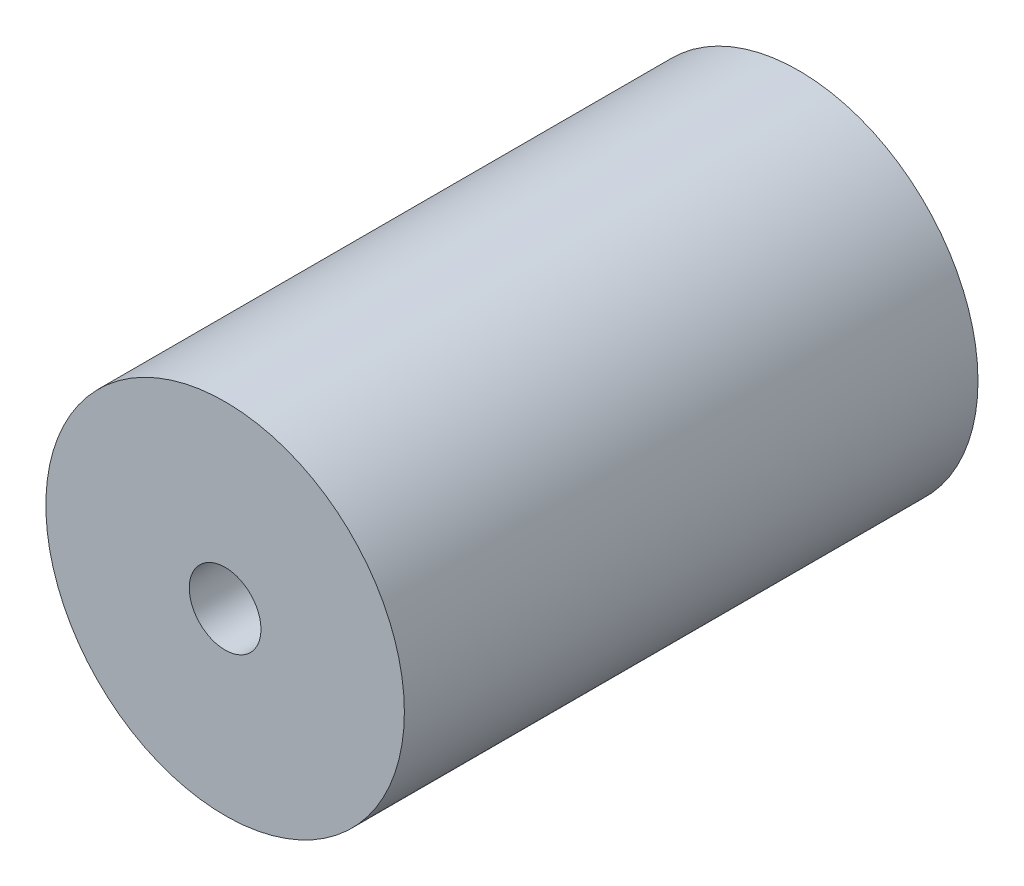
from build123d import *

# Parameters (mm, degrees)
SKETCH1_R           = 25
SKETCH1_R_2         = 5
BOSS_EXTRUDE1_DEPTH = 80


with BuildPart() as part:
    # Sketch1 → Boss-Extrude1 (new body)
    with BuildSketch(Plane.XY):
        Circle(SKETCH1_R)
        Circle(SKETCH1_R_2, mode=Mode.SUBTRACT)
    extrude(amount=BOSS_EXTRUDE1_DEPTH)


solid = part.part
